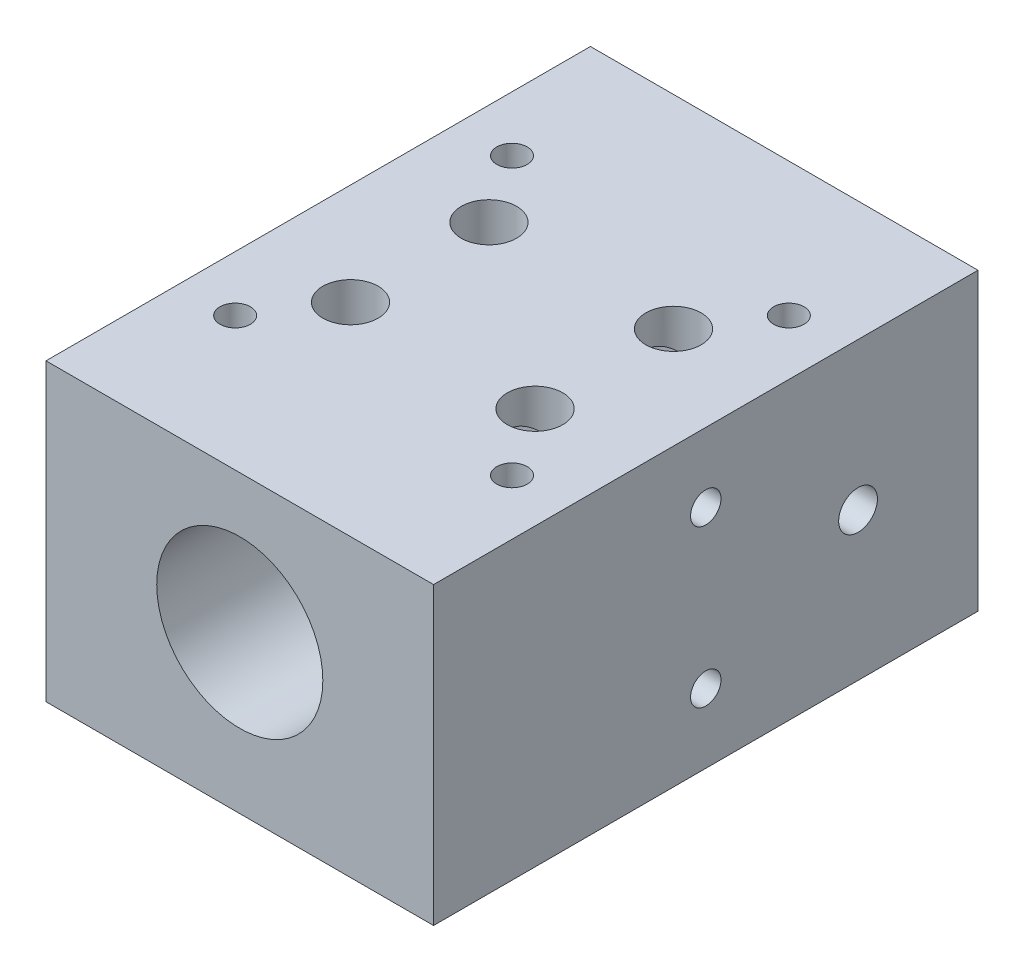
from build123d import *

# Parameters (mm, degrees)
SKETCH1_W                  = 42
SKETCH1_H                  = 32
SKETCH1_R                  = 9
BOSS_EXTRUDE1_DEPTH        = 59
SKETCH2_R                  = 13.5
CUT_EXTRUDE1_DEPTH         = 40
M4_TAPPED_HOLE1_AT_2_COUNT = 2
M4_TAPPED_HOLE1_AT_2_PITCH = 17
SKETCH8_R                  = 1.5
SKETCH8_R_2                = 3
CUT_EXTRUDE2_DEPTH         = 11
M4_TAPPED_HOLE2_D          = 3.3
M4_TAPPED_HOLE2_DEPTH      = 10
M4_TAPPED_HOLE2_TIP        = 0.991420021


with BuildPart() as part:
    # Sketch1 → Boss-Extrude1 (new body)
    with BuildSketch(Plane.XY):
        Rectangle(SKETCH1_W, SKETCH1_H)
        with Locations((0, 1)):
            Circle(SKETCH1_R, mode=Mode.SUBTRACT)
    extrude(amount=BOSS_EXTRUDE1_DEPTH)

    # Sketch2 → Cut-Extrude1 (cut)
    with BuildSketch(Plane(origin=(0, 0, 0), x_dir=(-1, 0, 0), z_dir=(0, 0, -1))):
        with Locations((0, 1)):
            Circle(SKETCH2_R)
    extrude(amount=-CUT_EXTRUDE1_DEPTH, mode=Mode.SUBTRACT)

    # Sketch4 → M4 Tapped Hole1 (revolve, cut)
    with BuildSketch(Plane(origin=(-21, 8.5, 29.5), x_dir=(0, 0, 1), z_dir=(0, 1, 0))):
        Polygon((0, 0), (0, 8.991420021), (1.65, 8), (1.65, 0), align=None)
    m4_tapped_hole1 = revolve(axis=Axis((-27.35, 8.5, 29.5), (1, 0, 0)), mode=Mode.SUBTRACT)

    # M4 Tapped Hole1 at 2: M4 Tapped Hole1 ×2
    with Locations(*[(0, -i * M4_TAPPED_HOLE1_AT_2_PITCH, 0) for i in range(1, M4_TAPPED_HOLE1_AT_2_COUNT)]):
        add(m4_tapped_hole1, mode=Mode.SUBTRACT)

    # Sketch6 → M5 Tapped Hole1 (revolve, cut)
    with BuildSketch(Plane(origin=(-21, 0, 13), x_dir=(0, 0, 1), z_dir=(0, 1, 0))):
        Polygon((0, 0), (0, 15.2618073), (2.1, 14), (2.1, 0), align=None)
    m5_tapped_hole1 = revolve(axis=Axis((-27.35, 0, 13), (1, 0, 0)), mode=Mode.SUBTRACT)

    # Mirror1: M4 Tapped Hole1, M5 Tapped Hole1 across plane
    add(m4_tapped_hole1.mirror(Plane(origin=(0, 0, 0), x_dir=(0, 0, 1), z_dir=(1, 0, 0))), mode=Mode.SUBTRACT)
    add(m5_tapped_hole1.mirror(Plane(origin=(0, 0, 0), x_dir=(0, 0, 1), z_dir=(1, 0, 0))), mode=Mode.SUBTRACT)

    # Mirror1 copy 1 sketch → Mirror1 copy 1 (revolve, cut)
    with BuildSketch(Plane(origin=(21, -8.5, 29.5), x_dir=(0, 0, 1), z_dir=(0, 1, 0))):
        Polygon((0, 0), (0, -8.991420021), (1.65, -8), (1.65, 0), align=None)
    revolve(axis=Axis((27.35, -8.5, 29.5), (1, 0, 0)), mode=Mode.SUBTRACT)

    # Sketch8 → Cut-Extrude2 (cut)
    with BuildSketch(Plane(origin=(0, 16, 0), x_dir=(1, 0, 0), z_dir=(0, 1, 0))):
        with Locations(Location((-15, -14.5, 0), (0, 0, 270))):
            Circle(SKETCH8_R)
        with Locations(Location((-10, -22, 0), (0, 0, 270))):
            Circle(SKETCH8_R_2)
        with Locations(Location((10, -22, 0), (0, 0, 270))):
            Circle(SKETCH8_R_2)
        with Locations(Location((15, -14.5, 0), (0, 0, 270))):
            Circle(SKETCH8_R)
        with Locations(Location((15, -44.5, 0), (0, 0, 90))):
            Circle(SKETCH8_R)
        with Locations(Location((10, -37, 0), (0, 0, 269.999992681))):
            Circle(SKETCH8_R_2)
        with Locations(Location((-10, -37, 0), (0, 0, 269.999954887))):
            Circle(SKETCH8_R_2)
        with Locations(Location((-15, -44.5, 0), (0, 0, 90))):
            Circle(SKETCH8_R)
    extrude(amount=-CUT_EXTRUDE2_DEPTH, mode=Mode.SUBTRACT)

    # M4 Tapped Hole2
    with Locations(Plane(origin=(0, 16, 0), x_dir=(1, 0, 0), z_dir=(0, 1, 0))):
        with Locations((15, -14.5), (15, -44.5), (-15, -44.5), (-15, -14.5)):
            Hole(M4_TAPPED_HOLE2_D / 2, depth=M4_TAPPED_HOLE2_DEPTH)
            with Locations((0, 0, -(M4_TAPPED_HOLE2_DEPTH + M4_TAPPED_HOLE2_TIP / 2))):  # 118° drill point
                Cone(0, M4_TAPPED_HOLE2_D / 2, M4_TAPPED_HOLE2_TIP, mode=Mode.SUBTRACT)


solid = part.part
